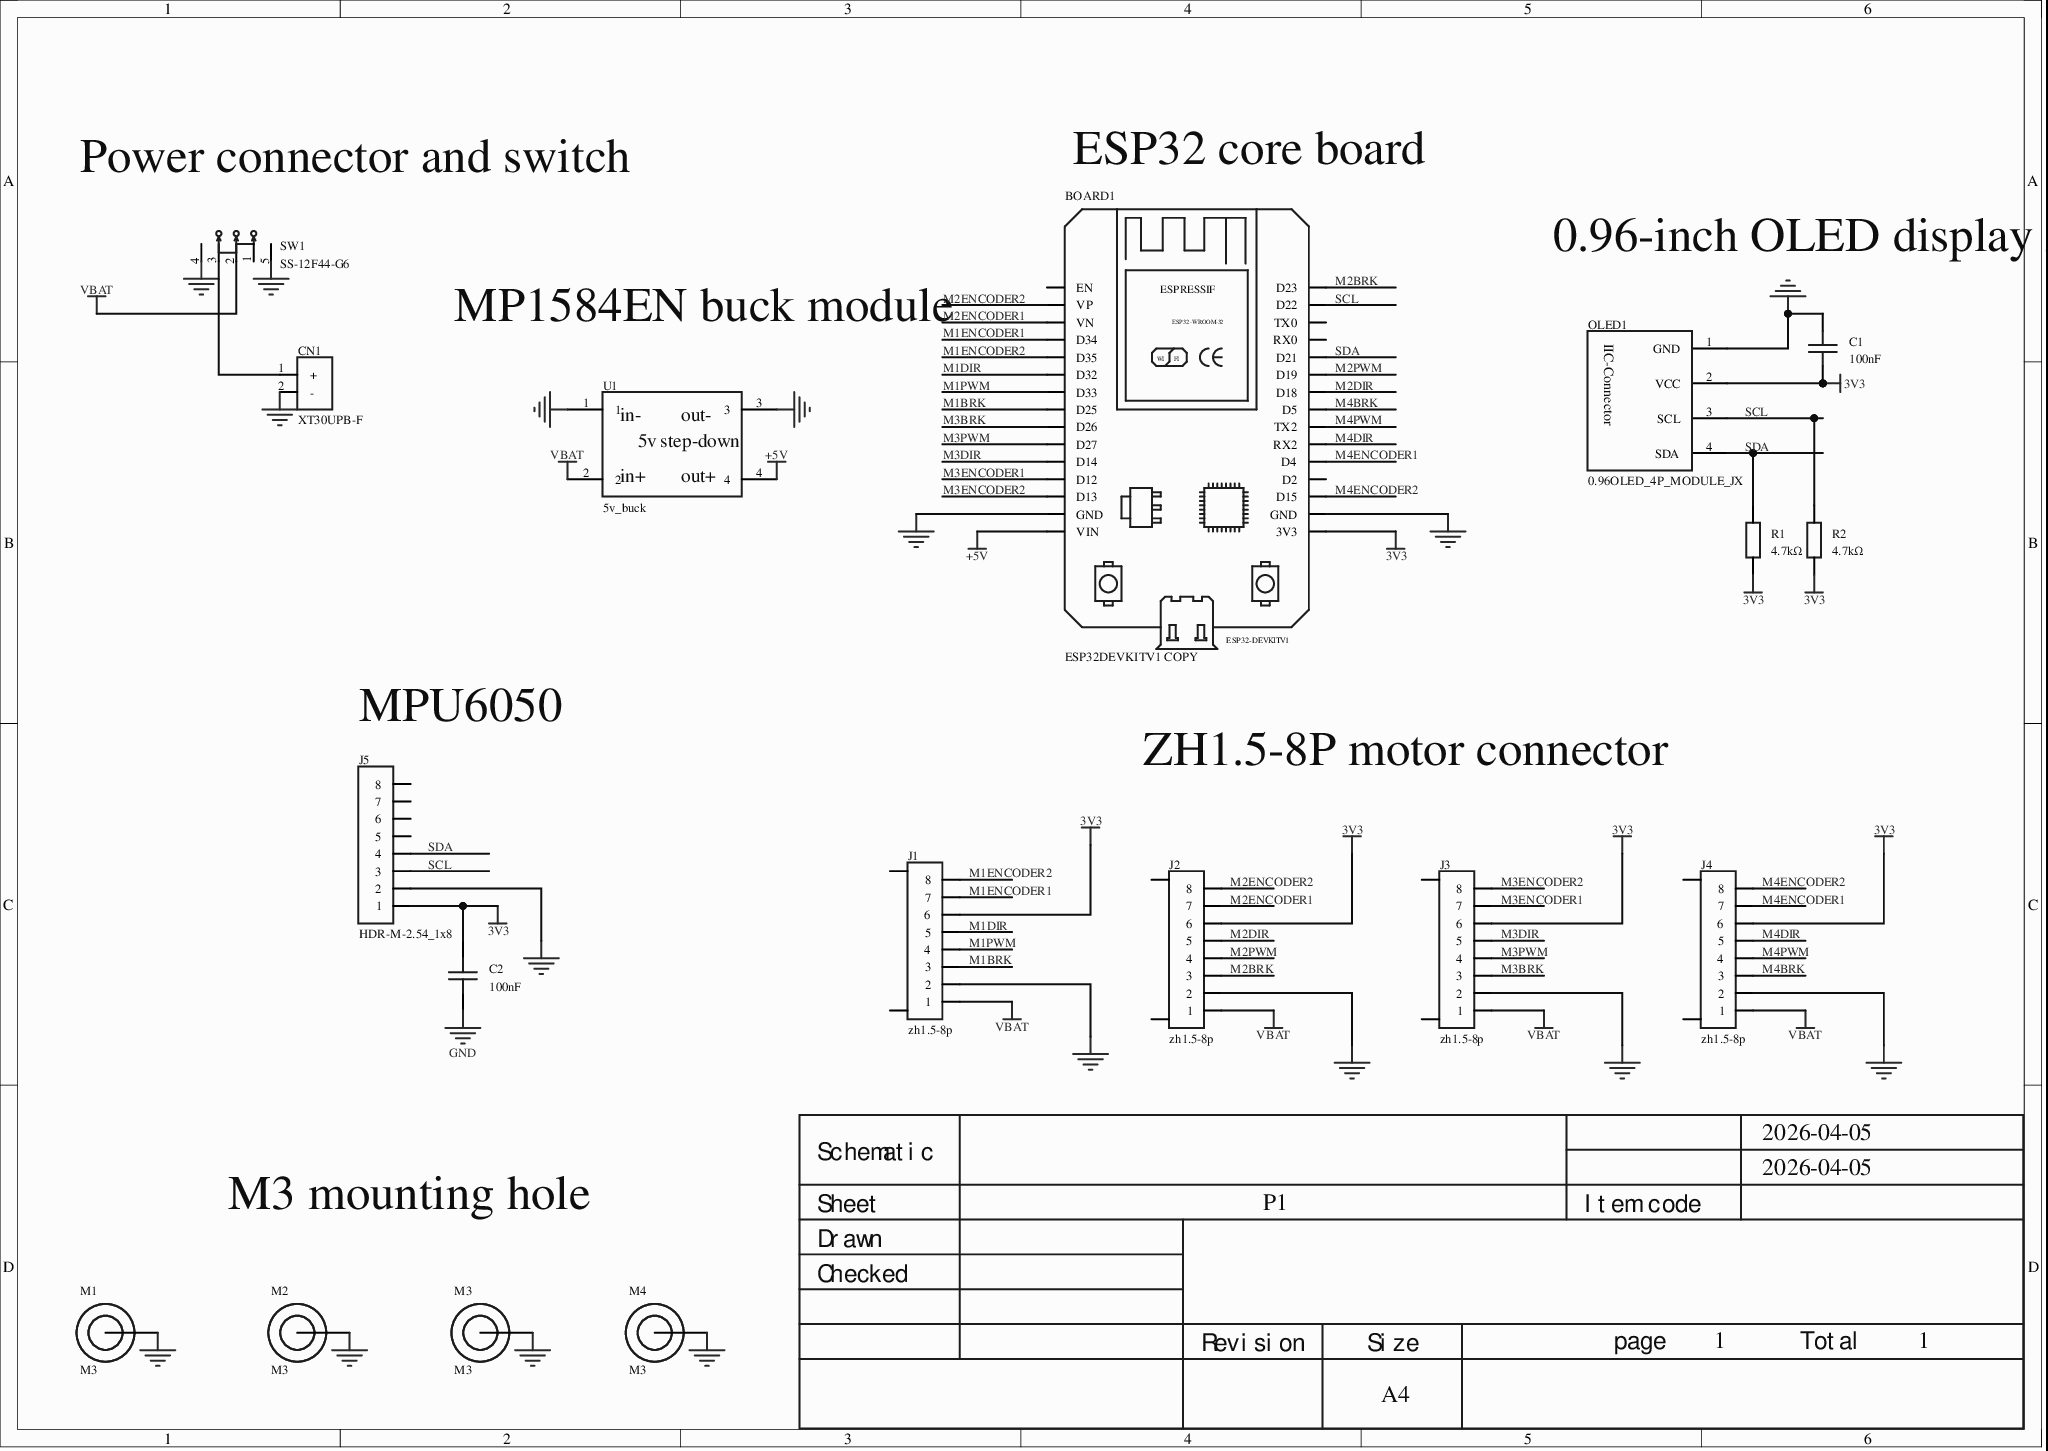
[diagram p0: MISC89094-3.schdoc]
# Altium project MISC89094-2.PrjPcb
1 sheet, 18 parts. Net scope: global (net labels, ports and power ports of the same name join across sheets).
Board file: MISC89094.pcbdoc

## Sheet MISC89094-3.schdoc
size 297 x 210 mm; Version: V1.0; @Project Name: MISC89094; @Page Count: 1; @Update Date: 2026-04-05; @Create Date: 2026-04-05; @Schematic Name: MISC89094; @Page No: 1

### Parts
BOARD1  ESP32DEVKITV1 COPY  [ESP32-DEVKITV1]
C1  100nF  [C0603]
C2  100nF  [C0603]
CN1  XT30UPB-F  [XT30]
J1  zh1.5-8p  [ZH1.5-8P]
J2  zh1.5-8p  [ZH1.5-8P]
J3  zh1.5-8p  [ZH1.5-8P]
J4  zh1.5-8p  [ZH1.5-8P]
J5  HDR-M-2.54_1x8  [HDR-M-2.54_1X8]
M1  M3  [M3]
M2  M3  [M3]
M3  M3  [M3]
M4  M3  [M3]
OLED1  0.96OLED_4P_MODULE_JX  [0.96OLED_4P]
R1  4.7kΩ  [Res_1/8W]
R2  4.7kΩ  [Res_1/8W]
SW1  SS-12F44-G6  [SW-TH_SS-12F44-GX]
U1  5v_buck  [5V_BUCK]

### Nets
3V3: BOARD1.3V3 C1.1 C2.2 J1.6 J2.6 J3.6 J4.6 J5.1 OLED1.2(VCC) R1.1 R2.1
+5V: BOARD1.VIN U1.4
GND: BOARD1.GND BOARD1.GND@1(GND) C1.2 C2.1 CN1.2(-) J1.2 J2.2 J3.2 J4.2 J5.2 M1.1 M2.1 M3.1 M4.1 OLED1.1(GND) SW1.4 SW1.5 U1.1 U1.3
VBAT: J1.1 J2.1 J3.1 J4.1 SW1.2 U1.2
M1BRK: BOARD1.D25 J1.3
M1DIR: BOARD1.D32 J1.5
M1ENCODER1: BOARD1.D34 J1.7
M1ENCODER2: BOARD1.D35 J1.8
M1PWM: BOARD1.D33 J1.4
M2BRK: BOARD1.D23 J2.3
M2DIR: BOARD1.D18 J2.5
M2ENCODER1: BOARD1.VN J2.7
M2ENCODER2: BOARD1.VP J2.8
M2PWM: BOARD1.D19 J2.4
M3BRK: BOARD1.D26 J3.3
M3DIR: BOARD1.D14 J3.5
M3ENCODER1: BOARD1.D12 J3.7
M3ENCODER2: BOARD1.D13 J3.8
M3PWM: BOARD1.D27 J3.4
M4BRK: BOARD1.D5 J4.3
M4DIR: BOARD1.RX2 J4.5
M4ENCODER1: BOARD1.D4 J4.7
M4ENCODER2: BOARD1.D15 J4.8
M4PWM: BOARD1.TX2 J4.4
SCL: BOARD1.D22 J5.3 OLED1.3(SCL) R2.2
SDA: BOARD1.D21 J5.4 OLED1.4(SDA) R1.2
NetCN1_1: CN1.1(+) SW1.3

Not connected (* = marked no-connect by the designer): BOARD1 D2* EN* RX0* TX0*; J1 9(10)* 10(9)*; J2 9(10)* 10(9)*; J3 9(10)* 10(9)*; J4 9(10)* 10(9)*; J5 5* 6* 7* 8*; SW1 1*

### Notes on the sheet
- (near SW1) Power connector and switch
- ESP32 core board
- 0.96-inch OLED display module
- MP1584EN buck module
- (near J5) MPU6050
- ZH1.5-8P motor connector
- M3 mounting hole
- 2026-04-05
- Schematic
- Sheet
- P1
- Item code
- Checked
- Drawn
- Revision
- Size
- A4
- page
- 1
- Total

### Library data of the parts
BOARD1 = ESP32DEVKITV1 COPY: AddInBom: yes; Device: ESP32DEVKITV1 COPY; ConvertToPcb: yes; SymbolName: ESP32DEVKITV1 COPY; FootprintName: ESP32-DEVKITV1
C1 C2 = CAP_0603: Symbol: Capacitance; ConvertToPcb: yes; ModelId: ac125912035d415993ca9572d50418b10819f05c4eef4c71ace90d822a990e87; ModelName: C0603_L1.6-W0.8-H0.8; ModelTransform: 62.992,31.496,0,0,0,0,0,0,0; Device: CAP_0603; AddInBom: yes; Supplier Footprint: 0603; FootprintName: C0603; Value: 100nF
CN1 = XT30: AddInBom: yes; Device: XT30; Symbol: XT30; ConvertToPcb: yes; FootprintName: XT30
J1-J4 = zh1.5-8p: AddInBom: yes; Device: zh1.5-8p; Symbol: zh1.5-8p; ConvertToPcb: yes; SupplierPart: C190820; Supplier: LCSC; FootprintName: ZH1.5-8P
J5 = HDR-M-2.54_1x8: AddInBom: yes; Device: HDR-M-2.54_1x8; Symbol: HDR-M-2.54_1x8; ConvertToPcb: yes; SupplierPart: C190820; Supplier: LCSC; FootprintName: HDR-M-2.54_1X8; JLCPCB Part Class: Extended library
M1-M4 = M3: AddInBom: yes; Device: M3; ConvertToPcb: yes; SymbolName: M3; FootprintName: M3
OLED1 = 0.96OLED_4P_MODULE_JX: Manufacturer: null; AddInBom: yes; Symbol: 0.96OLED_4P_MODULE_JX; Device: 0.96OLED_4P_MODULE_JX; Supplier: LCSC; Supplier Part: C9900004566; Manufacturer Part: 0.96OLED_4P_MODULE_JX; JLCPCB Part Class: Extended library; ConvertToPcb: yes; FootprintName: 0.96OLED_4P
R1 R2 = Res_AXIAL-1/8W: Symbol: Resistor; ConvertToPcb: yes; ModelId: b2b5ae7ae4c642178fe0039925c86a3f0819f05c4eef4c71ace90d822a990e87; ModelName: RES-TH_BD1.8-L3.2-P7.20-D0.4; ModelTransform: 282.86,66.88,253.09,0,0,0,0,0,-191; Device: Res_AXIAL-1/8W; Value: 4.7kΩ; AddInBom: yes; Supplier Footprint: 轴向引线; FootprintName: Res_1/8W
SW1 = SS-12F44-G6: Manufacturer: USAKRO; AddInBom: yes; Device: SS-12F44-G6; Symbol: SS-12F44-G6; ConvertToPcb: yes; Supplier: LCSC; SupplierPart: C698210; ManufacturerPart: SS-12F44-G6; JLCPCB Part Class: Extended library; FootprintName: SW-TH_SS-12F44-GX
U1 = 5v_buck: AddInBom: yes; Device: 5v_buck; Symbol: 5v_buck; ConvertToPcb: yes; FootprintName: 5V_BUCK